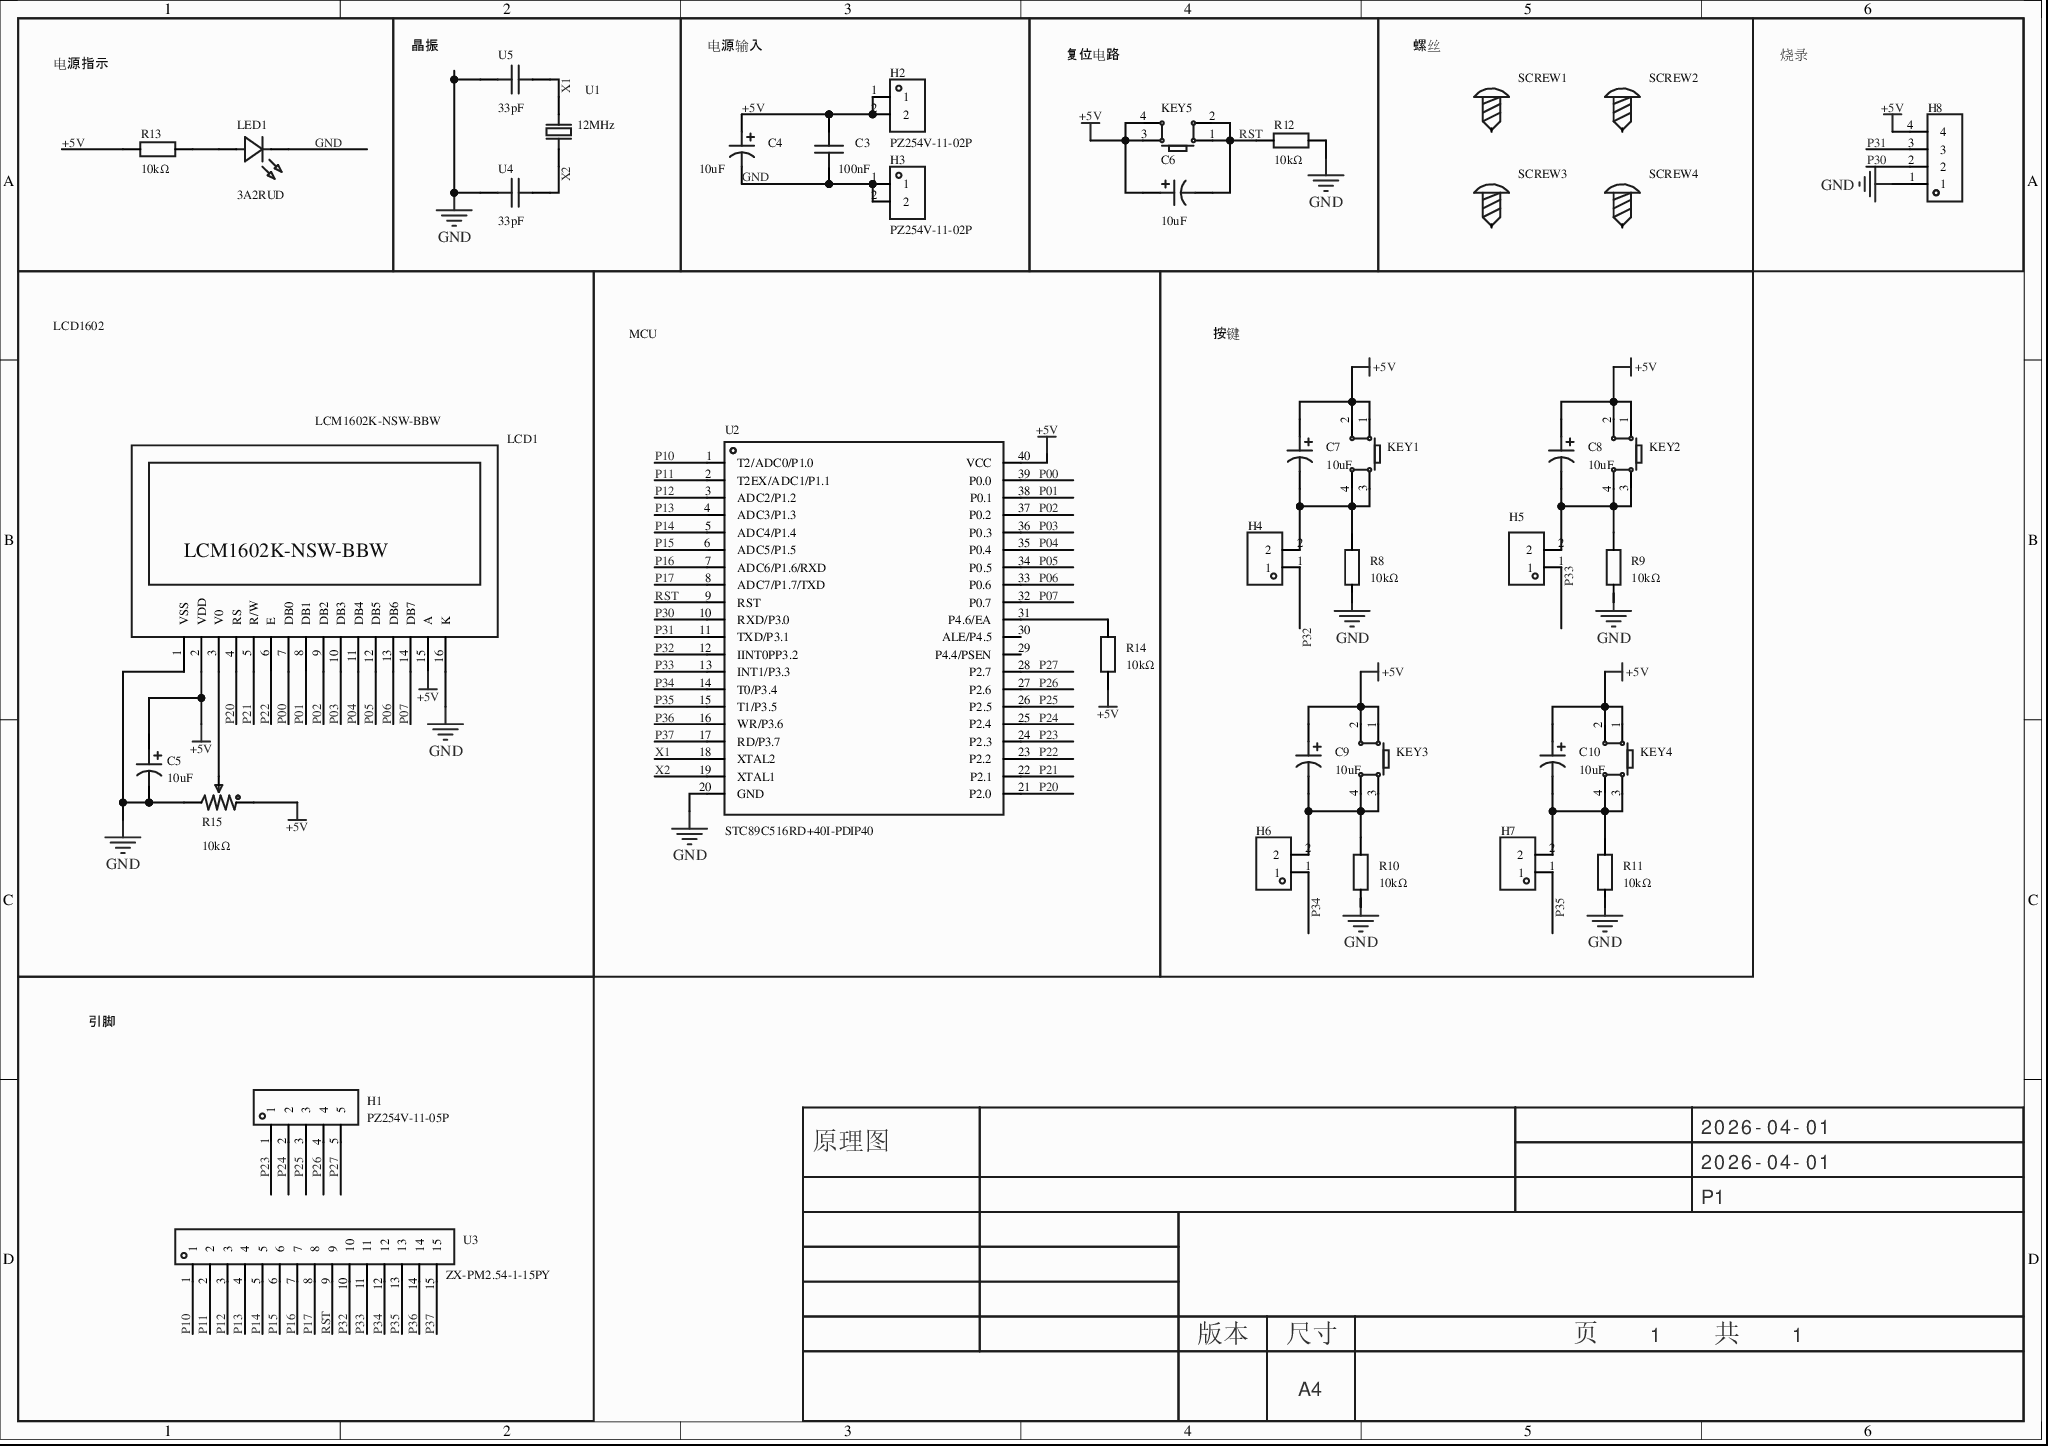
[diagram p0: MISC52019-3.schdoc]
# Altium project MISC52019-2.PrjPcb
1 sheet, 40 parts. Net scope: global (net labels, ports and power ports of the same name join across sheets).
Board file: MISC52019.pcbdoc

## Sheet MISC52019-3.schdoc
size 297 x 209 mm; Version: V1.0; @Project Name: MISC52019; @Page Count: 1; @Update Date: 2026-04-01; @Create Date: 2026-04-01; @Schematic Name: MISC52019; @Page No: 1; @Board Name: MISC52019; @Create Time: 18:47:32; @Update Time: 20:40:12; Size: A4

### Parts
C3  100nF  [CAP-TH_L5.0-W2.5-P5.00-D1.0]
C4  10uF  [CAP-TH_BD5.0-P2.00-D0.5-FD-A]
C5  10uF  [CAP-TH_BD5.0-P2.00-D0.5-FD-A]
C6  10uF  [CAP-TH_BD5.0-P2.00-D0.5-FD-A]
C7  10uF  [CAP-TH_BD5.0-P2.00-D0.5-FD-A]
C8  10uF  [CAP-TH_BD5.0-P2.00-D0.5-FD-A]
C9  10uF  [CAP-TH_BD5.0-P2.00-D0.5-FD-A]
C10  10uF  [CAP-TH_BD5.0-P2.00-D0.5-FD-A]
H1  PZ254V-11-05P  [HDR-TH_5P-P2.54-V-M]
H2  PZ254V-11-02P  [HDR-TH_2P-P2.54-V-M]
H3  PZ254V-11-02P  [HDR-TH_2P-P2.54-V-M]
H4  PZ254V-11-02P  [HDR-TH_2P-P2.54-V-M]  (value not drawn)
H5  PZ254V-11-02P  [HDR-TH_2P-P2.54-V-M]  (value not drawn)
H6  PZ254V-11-02P  [HDR-TH_2P-P2.54-V-M]  (value not drawn)
H7  PZ254V-11-02P  [HDR-TH_2P-P2.54-V-M]  (value not drawn)
H8  (no value)  [HDR-TH_4P-P2.54-V-F]
KEY1  (no value)  [SW-TH_4P-L6.0-W6.0-P4.50-LS6.5]
KEY2  (no value)  [SW-TH_4P-L6.0-W6.0-P4.50-LS6.5]
KEY3  (no value)  [SW-TH_4P-L6.0-W6.0-P4.50-LS6.5]
KEY4  (no value)  [SW-TH_4P-L6.0-W6.0-P4.50-LS6.5]
KEY5  (no value)  [SW-TH_4P-L6.0-W6.0-P4.50-LS6.5]
LCD1  LCM1602K-NSW-BBW  [MODULE-TH_LCM1602K]
LED1  3A2RUD  [LED-TH_BD3.5-P2.28_3A2RUC]
R8  10kΩ  [RES-TH_BD2.3-L6.5-P10.50-D0.5]
R9  10kΩ  [RES-TH_BD2.3-L6.5-P10.50-D0.5]
R10  10kΩ  [RES-TH_BD2.3-L6.5-P10.50-D0.5]
R11  10kΩ  [RES-TH_BD2.3-L6.5-P10.50-D0.5]
R12  10kΩ  [RES-TH_BD2.3-L6.5-P10.50-D0.5]
R13  10kΩ  [RES-TH_BD2.3-L6.5-P10.50-D0.5]
R14  10kΩ  [RES-TH_BD2.3-L6.5-P10.50-D0.5]
R15  10kΩ  [RES-ADJ-TH_3P-L10.0-W10.0-P2.50-L]
SCREW1  (no value)  [M2螺丝]
SCREW2  (no value)  [M2螺丝]
SCREW3  (no value)  [M2螺丝]
SCREW4  (no value)  [M2螺丝]
U1  12MHz  [HC-49S_L11.0-W4.7-P4.88]
U2  STC89C516RD+40I-PDIP40  [DIP-40_L52.3-W13.9-P2.54-LS15.2-BL]
U3  ZX-PM2.54-1-15PY  [HDR-TH_15P-P2.54-V-F]
U4  33pF  [CAP-TH_L5.0-W2.5-P5.08-D0.7]
U5  33pF  [CAP-TH_L5.0-W2.5-P5.08-D0.7]

### Blocks framed on the sheet
电源指示: LED1 R13
晶振: U1 U4 U5
电源输入: C3 C4 H2 H3
复位电路: C6 KEY5 R12
螺丝: SCREW1-SCREW4
烧录: H8
LCD1602: C5 LCD1 R15
MCU: R14 U2
按键: C7-C10 H4-H7 KEY1-KEY4 R8-R11
引脚: H1 U3

### Nets
+5V: C3.2 C4.1 C5.1 C6.1 C7.1 C8.1 C9.1 C10.1 H2.1 H2.2 H8.4 KEY1.1 KEY1.2 KEY2.1 KEY2.2 KEY3.1 KEY3.2 KEY4.1 KEY4.2 KEY5.3 KEY5.4 LCD1.2(VDD) LCD1.15(A) R13.2 R14.1 R15.1 U2.40(VCC)
GND: C3.1 C4.2 C5.2 H3.1 H3.2 H8.1 LCD1.1(VSS) LCD1.16(K) LED1.1(K) R8.1 R9.1 R10.1 R11.1 R12.1 R15.3 U2.20(GND) U4.1 U5.1
P00: LCD1.7(DB0) U2.39(P0.0)
P01: LCD1.8(DB1) U2.38(P0.1)
P02: LCD1.9(DB2) U2.37(P0.2)
P03: LCD1.10(DB3) U2.36(P0.3)
P04: LCD1.11(DB4) U2.35(P0.4)
P05: LCD1.12(DB5) U2.34(P0.5)
P06: LCD1.13(DB6) U2.33(P0.6)
P07: LCD1.14(DB7) U2.32(P0.7)
P10: U2.1(T2/ADC0/P1.0) U3.1
P11: U2.2(T2EX/ADC1/P1.1) U3.2
P12: U2.3(ADC2/P1.2) U3.3
P13: U2.4(ADC3/P1.3) U3.4
P14: U2.5(ADC4/P1.4) U3.5
P15: U2.6(ADC5/P1.5) U3.6
P16: U2.7(ADC6/P1.6/RXD) U3.7
P17: U2.8(ADC7/P1.7/TXD) U3.8
P20: LCD1.4(RS) U2.21(P2.0)
P21: LCD1.5(R/W) U2.22(P2.1)
P22: LCD1.6(E) U2.23(P2.2)
P23: H1.1 U2.24(P2.3)
P24: H1.2 U2.25(P2.4)
P25: H1.3 U2.26(P2.5)
P26: H1.4 U2.27(P2.6)
P27: H1.5 U2.28(P2.7)
P30: H8.2 U2.10(RXD/P3.0)
P31: H8.3 U2.11(TXD/P3.1)
P32: H4.1 U2.12(IINT0PP3.2) U3.10
P33: H5.1 U2.13(INT1/P3.3) U3.11
P34: H6.1 U2.14(T0/P3.4) U3.12
P35: H7.1 U2.15(T1/P3.5) U3.13
P36: U2.16(WR/P3.6) U3.14
P37: U2.17(RD/P3.7) U3.15
RST: C6.2 KEY5.1 KEY5.2 R12.2 U2.9(RST) U3.9
X1: U1.2 U2.18(XTAL2) U5.2
X2: U1.1 U2.19(XTAL1) U4.2
NetC7_2: C7.2 H4.2 KEY1.3 KEY1.4 R8.2
NetC8_2: C8.2 H5.2 KEY2.3 KEY2.4 R9.2
NetC9_2: C9.2 H6.2 KEY3.3 KEY3.4 R10.2
NetC10_2: C10.2 H7.2 KEY4.3 KEY4.4 R11.2
NetLCD1_3: LCD1.3(V0) R15.2
NetLED1_2: LED1.2(A) R13.1
NetR14_2: R14.2 U2.31(P4.6/EA)

Not connected (* = marked no-connect by the designer): SCREW1 1*; SCREW2 1*; SCREW3 1*; SCREW4 1*; U2 29(P4.4/PSEN)* 30(ALE/P4.5)*

### Notes on the sheet
- 2026-04-01
- 原理图
- P1
- 版本
- 尺寸
- A4
- 页    1    共    1

### Library data of the parts
C3 = CC1H104MC1FD3F6C10MF: 容值:100nF;精度:±20%;额定电压:50V;温度系数:Y5V;; Manufacturer: Dersonic(德尔创); AddInBom: yes; ModelId: 08e3d7481fc7486bb1b263873f51e1e1; ModelName: CAP-TH_BD5.0-W2.5-P5.08; ModelTransform: 224.652,98.425,0,0,0,0,-0.005,0,-137.795; Tolerance: ±20%; Voltage Rating: 50V; Pin Spacing: 5.08mm; Temperature Coefficient: Y5V; Body Thickness: 2.2mm; Symbol: CC1H104MC1FD3F6C10MF; Device: CC1H104MC1FD3F6C10MF; LCSC Part Name: 100nF ±20% 50V; SupplierPart: C254085; ManufacturerPart: CC1H104MC1FD3F6C10MF; Supplier Footprint: 插件,P=5.08mm; JLCPCB Part Class: 扩展库; Datasheet: https://item.szlcsc.com/datasheet/CC1H104MC1FD3F6C10MF/248635.html; Supplier: LCSC; ConvertToPcb: yes; FootprintName: CAP-TH_L5.0-W2.5-P5.00-D1.0; Value: 100nF; Diameter: 6mm
C4-C10 = ERG50V10M5X11: 容值:10uF;精度:±20%;额定电压:50V;纹波电流:180mA@100kHz;等效串联电阻(ESR):1.3Ω@100kHz;; Manufacturer: JIERR(捷而瑞); AddInBom: yes; ModelId: 230b3bd6484f4b52b9cf74c8bd6c6199; ModelTransform: 197.2437,197.23953,0,0,0,0,0,0,-196.85; Tolerance: ±20%; Voltage Rating: 50V; Pin Spacing: 2mm; Lifetime: 2000hrs@105℃; Symbol: ERG50V10M5X11; Device: ERG50V10M5X11; LCSC Part Name: 10uF ±20% 50V; SupplierPart: C47344184; ManufacturerPart: ERG50V10M5X11; Supplier Footprint: 插件,D5xL11mm; JLCPCB Part Class: 扩展库; Datasheet: https://item.szlcsc.com/datasheet/ERG50V10M5X11/49556625.html; Supplier: LCSC; ConvertToPcb: yes; FootprintName: CAP-TH_BD5.0-P2.00-D0.5-FD-A; ModelName: CAP-TH_BD5.0-P2.00-D0.5-FD-A; Value: 10uF; Ripple Current: 180mA@100kHz; Equivalent Series Resistance(ESR): 1.3Ω@100kHz; Diameter: 5mm; Height - Seated (Max): 11mm; Operating Temperature: -40℃~+105℃
H1 = PZ254V-11-05P: 插针结构:1x5P;间距:2.54mm;行距:-;圆针/方针:方针;安装方式:直插;排数:单排;总PIN位数:5P;额定电流:3A;额定电压:250V;配合针长度:6mm;塑高:2.5mm;端接针长度:3mm;触头材质:黄铜;触头镀层:-;工作温度:-40℃~+105℃;颜色:黑色;; Manufacturer: XFCN(兴飞); AddInBom: yes; ModelId: 47d466e4a34f4fc5bc626cf773a24dd5; ModelName: HDR-TH_5P-P2.54-M-LI-1X5P; ModelTransform: 499.999,100,0,0,0,0,0,0,-118.11; Pin Structure: 1x5P; Pitch: 2.54mm; Circluar Pins/Square Pins: 方针; Current Rating: 3A; Voltage Rating (Max): 250V; Symbol: PZ254V-11-05P; Device: PZ254V-11-05P; LCSC Part Name: 1x5P 间距:2.54mm 方针 直插; SupplierPart: C492404; ManufacturerPart: PZ254V-11-05P; Supplier Footprint: 插件,P=2.54mm; JLCPCB Part Class: 扩展库; Datasheet: https://item.szlcsc.com/datasheet/PZ254V-11-05P/502960.html; Supplier: LCSC; ConvertToPcb: yes; FootprintName: HDR-TH_5P-P2.54-V-M; Row Spacing: -; Mounting Type: 直插; Number of Rows: 单排; Number of Pins: 5P; Length of Mating Pin: 6mm; Insulation Height: 2.5mm; Length of End Connection Pin: 3mm; Contact Material: 黄铜; Contact Plating: -; Operating Temperature: -40℃~+105℃; Color: 黑色
H2-H7 = PZ254V-11-02P: 插针结构:1x2P;间距:2.54mm;行距:-;圆针/方针:方针;安装方式:直插;排数:单排;总PIN位数:2P;额定电流:3A;额定电压:250V;配合针长度:6mm;塑高:2.5mm;端接针长度:3mm;触头材质:黄铜;触头镀层:-;工作温度:-40℃~+105℃;颜色:黑色;; Manufacturer: XFCN(兴飞); AddInBom: yes; ModelId: e35305ec3aa84b66b849f914b715e73f; ModelName: HDR2.54-M-LI-1X2P; ModelTransform: 200,100,0,0,0,0,0,0,-118.11; Pin Structure: 1x2P; Pitch: 2.54mm; Circluar Pins/Square Pins: 方针; Current Rating: 3A; Voltage Rating (Max): 250V; Symbol: PZ254V-11-02P; Device: PZ254V-11-02P; LCSC Part Name: 1x2P 间距:2.54mm 方针 直插; SupplierPart: C492401; ManufacturerPart: PZ254V-11-02P; Supplier Footprint: 插件,P=2.54mm; JLCPCB Part Class: 扩展库; Datasheet: https://item.szlcsc.com/datasheet/PZ254V-11-02P/502957.html; Supplier: LCSC; ConvertToPcb: yes; FootprintName: HDR-TH_2P-P2.54-V-M; Row Spacing: -; Mounting Type: 直插; Number of Rows: 单排; Number of Pins: 2P; Length of Mating Pin: 6mm; Insulation Height: 2.5mm; Length of End Connection Pin: 3mm; Contact Material: 黄铜; Contact Plating: -; Operating Temperature: -40℃~+105℃; Color: 黑色
H8 = HDR-F_2.54_1x4P: Symbol: 2.54-1*4P母; ConvertToPcb: yes; ModelId: d187812051054f85879fcaa51a310d8e; ModelTransform: 419.6842,98.464,0,0,0,0,0,0,-118.11; Device: HDR-F_2.54_1x4P; AddInBom: yes; SupplierPart: C2718488; Supplier Footprint: 插件; FootprintName: HDR-TH_4P-P2.54-V-F; ModelName: HDR-TH_4P-P2.54-V-F
KEY1-KEY5 = Key_TH_6x6x6: 触点电流:50mA;额定电压(DC):12V;绝缘电阻:100MΩ;电路结构:单刀单掷;安装方式:直插;按钮形状:圆形按钮;按钮/盖帽颜色:黑色;作用力:260gf@±30gf;工作温度:-25℃~+70℃;引脚样式:PC引脚;开关长度:6mm;开关宽度:6mm;开关高度:6mm;带支架:否;; Symbol: 轻触按键; ConvertToPcb: yes; ModelId: 20eee248bc684ccd8cbdbb1d0d91ec6f; ModelName: SW-TH_4P-L6.0-W6.0-H5.0-LS6.5-P4.50; ModelTransform: 236.22,323.03,0,90,0,0,0,0,-137.795; Device: Key_TH_6x6x6; AddInBom: yes; SupplierPart: C2837516; Supplier Footprint: 插件; FootprintName: SW-TH_4P-L6.0-W6.0-P4.50-LS6.5
LCD1 = LCM1602K-NSW-BBW: 核心芯片:KS0066U;尺寸(inch):-;; Manufacturer: LONTECH(厦门龙特); AddInBom: yes; ModelId: 84dc4c036e12490da40aa0593fb5d02d; ModelTransform: 3149.6,1417.32,0,0,0,0,509.803,-610.157,0; Display Range: 64.5x16.4mm; Display Color: 蓝底白字; Voltage - Supply: 4.7V~5.5V；2.7V~5.3V; Symbol: LCM1602K-NSW-BBW; Device: LCM1602K-NSW-BBW; LCSC Part Name: LCM1602K-NSW-BBW; SupplierPart: C83275; ManufacturerPart: LCM1602K-NSW-BBW; Supplier Footprint: -; JLCPCB Part Class: 扩展库; Datasheet: https://item.szlcsc.com/datasheet/LCM1602K-NSW-BBW/84439.html; Supplier: LCSC; ConvertToPcb: yes; FootprintName: MODULE-TH_LCM1602K; ModelName: MODULE-TH_LCM1602K; Controller Type: KS0066U; Size: -
LED1 = 3A2RUD: 灯头类型:3mm圆形灯头;发光颜色:红色;正向压降(Vf):1.8V~2.2V;正向电流:20mA;波长:620nm~625nm;透镜颜色:红色透镜;色温:-;发光强度:200mcd~400mcd;发光角度:30°;工作温度:-40℃~+85℃;; Manufacturer: Guiguang light(桂光光电); AddInBom: yes; ModelId: 7dc1228e7ab44762a69569a9a69b2349; ModelTransform: 129.53171,137.754,0,0,0,0,-3.937,0,-196.85; Illumination Color: 红色; Forward Current: 20mA; Peak Wavelength: 625nm; Lens Color: 红色透镜; Viewing Angle: 30°; Symbol: 3A2RUD; Device: 3A2RUD; LCSC Part Name: 3mm 红发红短脚; SupplierPart: C52034637; ManufacturerPart: 3A2RUD; Supplier Footprint: 插件,D=3mm; JLCPCB Part Class: 扩展库; Datasheet: https://item.szlcsc.com/datasheet/3A2RUD/54791005.html; Supplier: LCSC; ConvertToPcb: yes; FootprintName: LED-TH_BD3.5-P2.28_3A2RUC; ModelName: LED-TH_BD3.5-P2.28_3A2RUC; Lamp Holder Type: 3mm圆形灯头; Voltage - Forward(Vf): 1.8V~2.2V; Wavelength - Dominant: 620nm~625nm; Color Temperature: -; Luminous Intensity: 200mcd~400mcd; Operating Temperature: -40℃~+85℃
R8-R14 = MF1/4W-10KΩ±1% T: 电阻类型:金属膜电阻;阻值:10kΩ;精度:±1%;功率:250mW;温度系数:±100ppm/℃;; Manufacturer: CCO(千志电子); Symbol: MF1/4W-10KΩ±1% T52; AddInBom: yes; ModelId: 8e6c7ee8323443d1ab8f0504b6353c8c; ModelName: RES-TH_D2.3-L6.5-P10.50; ModelTransform: 431.1015,91.3384,0,0,0,0,0.197,0,-137.795; Tolerance: ±1%; Voltage-Supply(Max): 250V; Power(Watts): 250mW; Device: MF1/4W-10KΩ±1% T; LCSC Part Name: 10kΩ ±1% 250mW 金属膜电阻 圆柱状直插; SupplierPart: C119347; ManufacturerPart: MF1/4W-10KΩ±1% T; Supplier Footprint: 插件,D2.3xL6.5mm; JLCPCB Part Class: 扩展库; Datasheet: https://atta.szlcsc.com/upload/public/pdf/source/20190910/C427326_62A6D058BC0FF74963A2F22379CA06CE.pdf; Supplier: LCSC; ConvertToPcb: yes; FootprintName: RES-TH_BD2.3-L6.5-P10.50-D0.5; Type: 金属膜电阻; Value: 10kΩ; Temperature Coefficient: ±100ppm/℃; Operating Temperature: -55℃~+155℃
R15 = 3296W-1-103: 阻值:10kΩ;精度:±10%;功率:500mW;温度系数:±250ppm/℃;; Manufacturer: BOCHEN(博晨); AddInBom: yes; ModelId: b182808559bb43bda9e7de64b64134cb; ModelName: 3296W; ModelTransform: 374.015,188.976,0,180,0,0,0,0,-137.795; Tolerance: ±10%; Power(Watts): 500mW; Number of Turns: 30; Symbol: 3296W-1-103; Device: 3296W-1-103; LCSC Part Name: 10kΩ ±10%; SupplierPart: C118954; ManufacturerPart: 3296W-1-103; Supplier Footprint: 插件-3P,9.5x4.9mm; JLCPCB Part Class: 扩展库; Datasheet: https://item.szlcsc.com/datasheet/3296W-1-103/120223.html; Supplier: LCSC; ConvertToPcb: yes; FootprintName: RES-ADJ-TH_3P-L10.0-W10.0-P2.50-L; Value: 10kΩ; Temperature Coefficient: ±250ppm/℃
SCREW1-SCREW4 = M2螺丝: ConvertToPcb: yes; SymbolName: 螺丝孔; Device: M2螺丝; AddInBom: yes; Supplier Footprint: 插件; FootprintName: M2螺丝
U1 = YG12MLBBE2X: 晶振类型:插件晶振;频率:12MHz;常温频差:±10ppm;负载电容:20pF;频率稳定度:±30ppm;; Manufacturer: YJX(雅晶鑫); AddInBom: yes; ModelId: 90d89857b3344bee9813507fec06adb2; ModelTransform: 435.0385,183.0705,0,0,0,0,0,0,-196.85; Normal temperature Frequency Tolerance: ±10ppm; Load Capacitance: 20pF; Frequency Stability: ±30ppm; Equivalent Series Resistance(ESR): 40Ω; Symbol: YG12MLBBE2X; Device: YG12MLBBE2X; LCSC Part Name: 49S 12M 20PF 10PPM; SupplierPart: C42441036; ManufacturerPart: YG12MLBBE2X; Supplier Footprint: HC-49S; Datasheet: https://atta.szlcsc.com/upload/public/pdf/source/20250109/7D5687D7E6E611B127181E4BD00ED56D.pdf; Supplier: LCSC; ConvertToPcb: yes; FootprintName: HC-49S_L11.0-W4.7-P4.88; ModelName: HC-49S_L11.0-W4.7-P4.88; Type: 插件晶振; Value: 12MHz; Operating Temperature: -20℃~+70℃
U2 = STC89C516RD+40I-PDIP40: CPU内核:51系列;应用领域:-;; Manufacturer: STC; AddInBom: yes; ModelId: 16d4686a009b4ddca948f91eddb57b14; ModelName: DIP-40_L52.3-W13.8-H4.0-LS15.24-P2.54; ModelTransform: 2059.051,615.743,0,0,0,0,0,0,-129.921; CPU Core: 51系列; Program Storage Size: 61KB; Program Memory Type: FLASH; Number of I/O: 35; Voltage - Supply: 3.5V~5.5V; Symbol: STC89C516RD+40I-PDIP40; Device: STC89C516RD+40I-PDIP40; LCSC Part Name: STC89C516RD+40I-PDIP40; SupplierPart: C52225; ManufacturerPart: STC89C516RD+40I-PDIP40; Supplier Footprint: DIP-40; JLCPCB Part Class: 扩展库; Datasheet: https://atta.szlcsc.com/upload/public/pdf/source/20250219/C2F0DDDE7C5E9ADA5B33742D18630F09.pdf; Supplier: LCSC; ConvertToPcb: yes; FootprintName: DIP-40_L52.3-W13.9-P2.54-LS15.2-BL; Applications: -
U3 = ZX-PM2.54-1-15PY: 插孔结构:1x15P;间距:2.54mm;行距:-;圆孔/方孔:方孔;安装方式:直插;排数:单排;总孔位数:15P;额定电流:3A;额定电压:-;插孔方向:顶部;塑高:8.5mm;触头材质:黄铜;触头镀层:金;工作温度:-40℃~+105℃;; Manufacturer: Megastar(兆星); AddInBom: yes; ModelId: 38ff91cb466b435b8c8f2ba8086ca4a0; ModelTransform: 1515.745,98.425,0,0,0,0,0,0,-125.984; Holes Structure: 1x15P; Pitch: 2.54mm; Circular Hole / Square Hole: 方孔; Number of Positions: 15P; Current Rating: 3A; Holes Direction: 顶部; PIN Length: 3.2mm; Symbol: ZX-PM2.54-1-15PY; Device: ZX-PM2.54-1-15PY; LCSC Part Name: 1x15P 间距:2.54mm 直插; SupplierPart: C7499333; ManufacturerPart: ZX-PM2.54-1-15PY; Supplier Footprint: 插件,P=2.54mm; JLCPCB Part Class: 扩展库; Datasheet: https://item.szlcsc.com/datasheet/ZX-PM2.54-1-15PY/8573994.html; Supplier: LCSC; ConvertToPcb: yes; FootprintName: HDR-TH_15P-P2.54-V-F; ModelName: HDR-TH_15P-P2.54-V-F; Row Spacing: -; Mounting Type: 直插; Number of Rows: 单排; Voltage Rating (Max): -; Insulation Height: 8.5mm; Contact Material: 黄铜; Contact Plating: 金; Operating Temperature: -40℃~+105℃
U4 U5 = CC1H330JC74DCH4B10MN: 容值:33pF;精度:±5%;额定电压:50V;温度系数:NP0;; Manufacturer: Dersonic(德尔创); AddInBom: yes; ModelId: 3d005bb2736f4b028b929daf59d2a504; ModelName: CAP-TH_L5.0-W2.5-P5.08; ModelTransform: 222.8342,98.419,0,0,0,0,0,0,-118.11; Tolerance: ±5%; Voltage Rating: 50V; Pin Spacing: 5.08mm; Temperature Coefficient: NP0; Body Thickness: 2.2mm; Symbol: CC1H330JC74DCH4B10MN; Device: CC1H330JC74DCH4B10MN; LCSC Part Name: 33pF ±5% 50V; SupplierPart: C254101; ManufacturerPart: CC1H330JC74DCH4B10MN; Supplier Footprint: 插件,P=5.08mm; JLCPCB Part Class: 扩展库; Datasheet: https://item.szlcsc.com/datasheet/CC1H330JC74DCH4B10MN/248651.html; Supplier: LCSC; ConvertToPcb: yes; FootprintName: CAP-TH_L5.0-W2.5-P5.08-D0.7; Value: 33pF; Diameter: 4.7mm